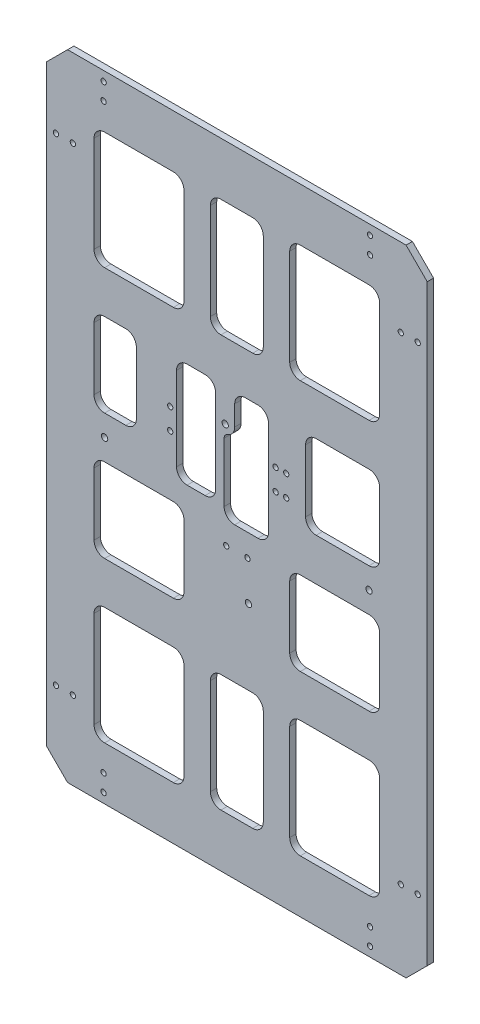
SolidWorks part; units mm, degrees
ref_plane "前视基准面" through (0, 0, 0) normal (0, 0, 1) x (1, 0, 0)
ref_plane "上视基准面" through (0, 0, 0) normal (0, 1, 0) x (1, 0, 0)
ref_plane "右视基准面" through (0, 0, 0) normal (1, 0, 0) x (0, 0, -1)
ref_plane "基准面4" through (0, 0, 0) normal (0, 0, -1) x (-1, 0, 0)
sketch "草图1" plane through (0, 0, 0) normal (0, 0, -1) x (-1, 0, 0)
  line L0 (20, 10) -> (20, 89.043)
  line L1 (30, 99.043) -> (47, 99.043)
  line L2 (57, 89.043) -> (57, 10)
  line L3 (47, 0) -> (30, 0)
  line L4 (2, -10) -> (-20, -10)
  line L5 (-30, 0) -> (-30, 89.043)
  line L6 (-20, 99.043) -> (-8, 99.043)
  line L7 (2, 89.043) -> (2, 70.043)
  line L8 (12, 55.9008) -> (12, 0)
  line L9 (95, 30) -> (95, 89.043)
  line L10 (105, 99.043) -> (125, 99.043)
  line L11 (135, 89.043) -> (135, 30)
  line L12 (125, 20) -> (105, 20)
  line L13 (125, -250) -> (60, -250)
  line L14 (50, -240) -> (50, -149.043)
  line L15 (60, -139.043) -> (125, -139.043)
  line L16 (135, -149.043) -> (135, -240)
  line L17 (50, 149.043) -> (50, 240)
  line L18 (60, 250) -> (125, 250)
  line L19 (135, 240) -> (135, 149.043)
  line L20 (125, 139.043) -> (60, 139.043)
  line L21 (15, 139.043) -> (-15, 139.043)
  line L22 (-25, 149.043) -> (-25, 240)
  line L23 (-15, 250) -> (15, 250)
  line L24 (25, 240) -> (25, 149.043)
  line L25 (-15, -139.043) -> (15, -139.043)
  line L26 (25, -149.043) -> (25, -240)
  line L27 (15, -250) -> (-15, -250)
  line L28 (-25, -240) -> (-25, -149.043)
  line L29 (-50, -30) -> (-50, -89.043)
  line L30 (-60, -99.043) -> (-125, -99.043)
  line L31 (-135, -89.043) -> (-135, -30)
  line L32 (-125, -20) -> (-60, -20)
  line L33 (-50, -149.043) -> (-50, -240)
  line L34 (-60, -250) -> (-125, -250)
  line L35 (-135, -240) -> (-135, -149.043)
  line L36 (-125, -139.043) -> (-60, -139.043)
  line L37 (-75, 20) -> (-125, 20)
  line L38 (-135, 30) -> (-135, 89.043)
  line L39 (-125, 99.043) -> (-75, 99.043)
  line L40 (-65, 89.043) -> (-65, 30)
  line L41 (60, -20) -> (125, -20)
  line L42 (135, -30) -> (135, -89.043)
  line L43 (125, -99.043) -> (60, -99.043)
  line L44 (50, -89.043) -> (50, -30)
  line L45 (-125, 250) -> (-60, 250)
  line L46 (-50, 240) -> (-50, 149.043)
  line L47 (-60, 139.043) -> (-125, 139.043)
  line L48 (-135, 149.043) -> (-135, 240)
  line L49 (160, -300) -> (180, -280)
  line L50 (180, -280) -> (180, 280)
  line L51 (180, 280) -> (160, 300)
  line L52 (160, 300) -> (-160, 300)
  line L53 (-160, 300) -> (-180, 280)
  line L54 (-180, 280) -> (-180, -280)
  line L55 (-180, -280) -> (-160, -300)
  line L56 (-160, -300) -> (160, -300)
  circle A0 centre (-36.6729, 56.4) radius 2.5
  circle A1 centre (-10, -31.1729) radius 2.5
  circle A2 centre (10, -31.1729) radius 2.5
  circle A3 centre (-171, 225.9659) radius 2.5
  circle A4 centre (-155, 225.9659) radius 2.5
  circle A5 centre (-125.9659, 275) radius 2.5
  circle A6 centre (-125.8998, 291) radius 2.5
  circle A7 centre (-171, -225.9022) radius 2.5
  circle A8 centre (-155, -225.9022) radius 2.5
  circle A9 centre (-125.9659, -275.0005) radius 2.5
  circle A10 centre (-125.9659, -291.0005) radius 2.5
  circle A11 centre (125.8998, 291) radius 2.5
  circle A12 centre (125.9659, 275) radius 2.5
  circle A13 centre (171, 225.9659) radius 2.5
  circle A14 centre (155, 225.9659) radius 2.5
  circle A15 centre (171, -225.9022) radius 2.5
  circle A16 centre (155, -225.9022) radius 2.5
  circle A17 centre (125.9659, -291.0005) radius 2.5
  circle A18 centre (125.9659, -275.0005) radius 2.5
  circle A19 centre (63, 56.4) radius 2.5
  circle A20 centre (63, 36.4) radius 2.5
  arc A21 (30, 0) -> (20, 10) centre (30, 10) cw
  arc A22 (20, 89.043) -> (30, 99.043) centre (30, 89.043) cw
  arc A23 (47, 99.043) -> (57, 89.043) centre (47, 89.043) cw
  arc A24 (57, 10) -> (47, 0) centre (47, 10) cw
  circle A25 centre (-46.6729, 56.4) radius 2.5
  circle A26 centre (-46.6729, 36.4) radius 2.5
  arc A27 (12, 0) -> (2, -10) centre (2, 0) cw
  arc A28 (-20, -10) -> (-30, 0) centre (-20, 0) cw
  arc A29 (-30, 89.043) -> (-20, 99.043) centre (-20, 89.043) cw
  arc A30 (-8, 99.043) -> (2, 89.043) centre (-8, 89.043) cw
  arc A31 (2, 70.043) -> (8.6667, 60.6149) centre (12, 70.043) ccw
  arc A32 (8.6667, 60.6149) -> (12, 55.9008) centre (7, 55.9008) cw
  circle A33 centre (-11, -68) radius 3
  circle A34 centre (11, 68) radius 3
  arc A35 (105, 20) -> (95, 30) centre (105, 30) cw
  arc A36 (95, 89.043) -> (105, 99.043) centre (105, 89.043) cw
  arc A37 (125, 99.043) -> (135, 89.043) centre (125, 89.043) cw
  arc A38 (135, 30) -> (125, 20) centre (125, 30) cw
  arc A39 (135, -240) -> (125, -250) centre (125, -240) cw
  arc A40 (60, -250) -> (50, -240) centre (60, -240) cw
  arc A41 (50, -149.043) -> (60, -139.043) centre (60, -149.043) cw
  arc A42 (125, -139.043) -> (135, -149.043) centre (125, -149.043) cw
  arc A43 (60, 139.043) -> (50, 149.043) centre (60, 149.043) cw
  arc A44 (50, 240) -> (60, 250) centre (60, 240) cw
  arc A45 (125, 250) -> (135, 240) centre (125, 240) cw
  arc A46 (135, 149.043) -> (125, 139.043) centre (125, 149.043) cw
  arc A47 (25, 149.043) -> (15, 139.043) centre (15, 149.043) cw
  arc A48 (-15, 139.043) -> (-25, 149.043) centre (-15, 149.043) cw
  arc A49 (-25, 240) -> (-15, 250) centre (-15, 240) cw
  arc A50 (15, 250) -> (25, 240) centre (15, 240) cw
  arc A51 (-25, -149.043) -> (-15, -139.043) centre (-15, -149.043) cw
  arc A52 (15, -139.043) -> (25, -149.043) centre (15, -149.043) cw
  arc A53 (25, -240) -> (15, -250) centre (15, -240) cw
  arc A54 (-15, -250) -> (-25, -240) centre (-15, -240) cw
  arc A55 (-60, -20) -> (-50, -30) centre (-60, -30) cw
  arc A56 (-50, -89.043) -> (-60, -99.043) centre (-60, -89.043) cw
  arc A57 (-125, -99.043) -> (-135, -89.043) centre (-125, -89.043) cw
  arc A58 (-135, -30) -> (-125, -20) centre (-125, -30) cw
  arc A59 (-60, -139.043) -> (-50, -149.043) centre (-60, -149.043) cw
  arc A60 (-50, -240) -> (-60, -250) centre (-60, -240) cw
  arc A61 (-125, -250) -> (-135, -240) centre (-125, -240) cw
  arc A62 (-135, -149.043) -> (-125, -139.043) centre (-125, -149.043) cw
  arc A63 (-65, 30) -> (-75, 20) centre (-75, 30) cw
  arc A64 (-125, 20) -> (-135, 30) centre (-125, 30) cw
  arc A65 (-135, 89.043) -> (-125, 99.043) centre (-125, 89.043) cw
  arc A66 (-75, 99.043) -> (-65, 89.043) centre (-75, 89.043) cw
  arc A67 (50, -30) -> (60, -20) centre (60, -30) cw
  arc A68 (125, -20) -> (135, -30) centre (125, -30) cw
  arc A69 (135, -89.043) -> (125, -99.043) centre (125, -89.043) cw
  arc A70 (60, -99.043) -> (50, -89.043) centre (60, -89.043) cw
  arc A71 (-135, 240) -> (-125, 250) centre (-125, 240) cw
  arc A72 (-60, 250) -> (-50, 240) centre (-60, 240) cw
  arc A73 (-50, 149.043) -> (-60, 139.043) centre (-60, 149.043) cw
  arc A74 (-125, 139.043) -> (-135, 149.043) centre (-125, 149.043) cw
  circle A75 centre (-125, 0) radius 3
  circle A76 centre (125, 0) radius 3
  circle A77 centre (-36.6729, 36.4) radius 2.5
extrude "凸台-拉伸1" add sketch "草图1" against normal blind 6
